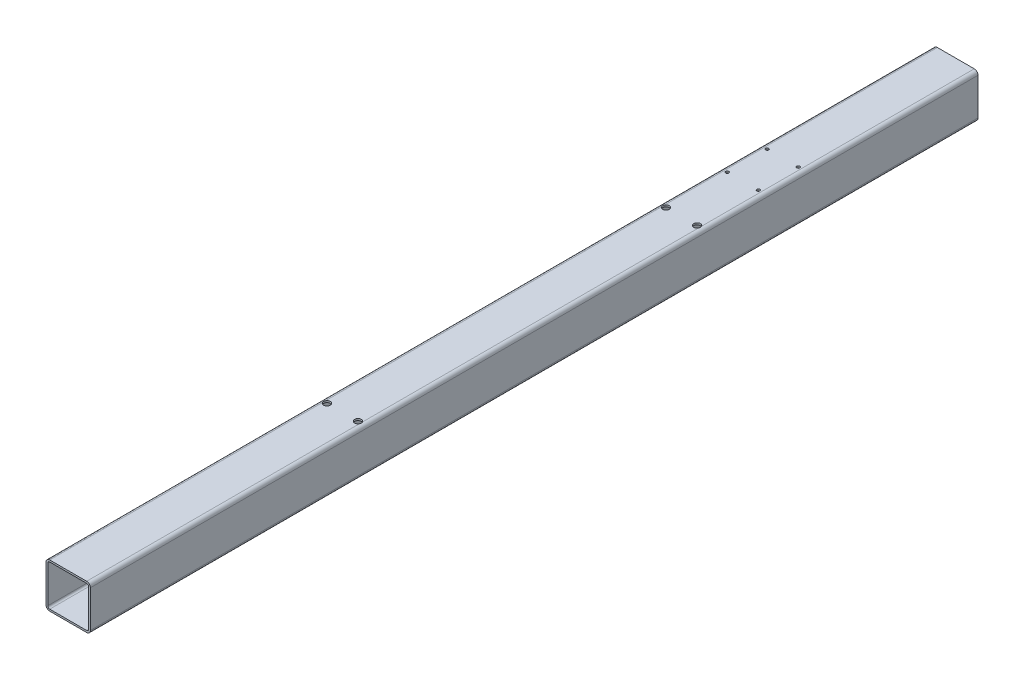
from build123d import *

# Parameters (mm, degrees)
SKETCH1_W             = 100
SKETCH1_H             = 100
BOSS_EXTRUDE1_DEPTH   = 2000
FILLET1_R             = 8.4
SHELL1_T              = -4
M8_TAPPED_HOLE1_D     = 6.8
M8_TAPPED_HOLE1_DEPTH = 19.75
M8_TAPPED_HOLE1_TIP   = 2.042926105
SKETCH2_R             = 7.5
SKETCH2_R_2           = 3
CUT_EXTRUDE1_DEPTH    = 10


with BuildPart() as part:
    # Sketch1 → Boss-Extrude1 (new body)
    with BuildSketch(Plane.XY):
        Rectangle(SKETCH1_W, SKETCH1_H)
    extrude(amount=BOSS_EXTRUDE1_DEPTH)

    # Fillet1
    fillet1_edges = [part.edges().sort_by_distance(p)[0] for p in [
        (-50, 50, 1000),
        (50, 50, 1000),
        (50, -50, 1000),
        (-50, -50, 1000),
    ]]
    fillet(fillet1_edges, radius=FILLET1_R)

    # Shell1
    shell1_openings = [part.faces().sort_by_distance(p)[0] for p in [
        (0, 0, 2000),
        (0, 0, 0),
    ]]
    offset(amount=SHELL1_T, openings=shell1_openings, kind=Kind.INTERSECTION)

    # M8 Tapped Hole1
    with Locations(Plane(origin=(0, 50, 0), x_dir=(1, 0, 0), z_dir=(0, 1, 0))):
        with Locations((-35, -390), (35, -390), (35, -480), (-35, -480)):
            Hole(M8_TAPPED_HOLE1_D / 2, depth=M8_TAPPED_HOLE1_DEPTH)
            with Locations((0, 0, -(M8_TAPPED_HOLE1_DEPTH + M8_TAPPED_HOLE1_TIP / 2))):  # 118° drill point
                Cone(0, M8_TAPPED_HOLE1_D / 2, M8_TAPPED_HOLE1_TIP, mode=Mode.SUBTRACT)

    # Sketch2 → Cut-Extrude1 (cut)
    with BuildSketch(Plane(origin=(0, 50, 0), x_dir=(1, 0, 0), z_dir=(0, 1, 0))):
        with Locations(Location((35, -618, 0), (0, 0, 331.642363424))):
            Circle(SKETCH2_R)
        with Locations(Location((-35, -618, 0), (0, 0, 208.357636576))):
            Circle(SKETCH2_R)
        with Locations(Location((35, -1382, 0), (0, 0, 331.642363424))):
            Circle(SKETCH2_R)
        with Locations(Location((-35, -1382, 0), (0, 0, 208.357636576))):
            Circle(SKETCH2_R)
        with Locations((-35, -390)):
            Circle(SKETCH2_R_2)
        with Locations((35, -390)):
            Circle(SKETCH2_R_2)
        with Locations((35, -480)):
            Circle(SKETCH2_R_2)
        with Locations((-35, -480)):
            Circle(SKETCH2_R_2)
    extrude(amount=-CUT_EXTRUDE1_DEPTH, mode=Mode.SUBTRACT)


solid = part.part
